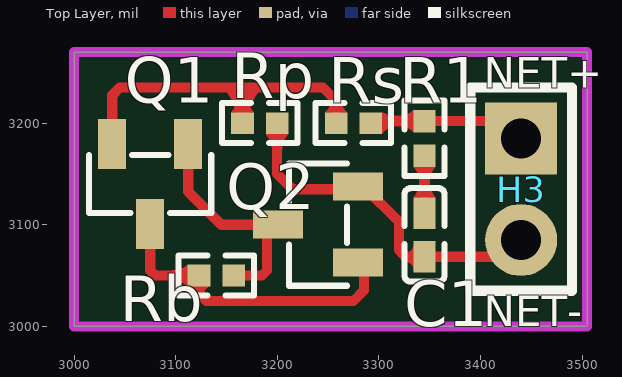
[diagram p0: Top Layer view]
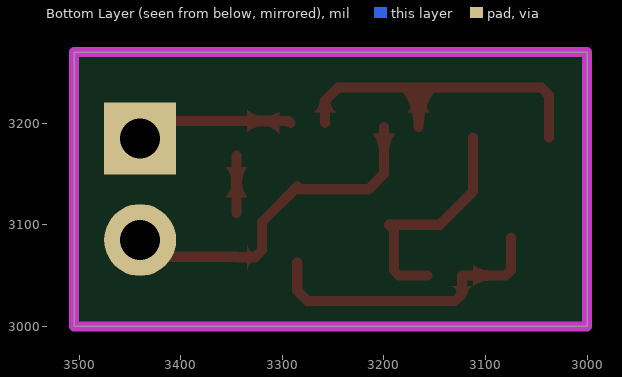
[diagram p1: Bottom Layer view, seen from below]
# Altium PCB MISC51453.pcbdoc
Units mil, origin at the board's own origin, x right, y up, seen from the top; angles counter-clockwise.
Board outline 505 x 270 mil, 2 copper layers (Top Layer, Bottom Layer), stack 62.206 mil thick; 8 components, 6 nets, 18 pads, 0 vias.

## Layer stack, top to bottom
Top Solder Mask Layer: solder mask 0.394, Dk 3.3
Top Layer: signal copper 1.379
Dielectric1: surface 59.449, FR4, Dk 4.5
Bottom Layer: signal copper 1.378
Bottom Solder Mask Layer: solder mask 0.394, Dk 3.3

## Board outline
3000,3270 3000,3000 3505,3000 3505,3270

## Design rules (kind name [scope] priority, off if disabled: settings)
BoardOutlineClearance copperThickness2oz_1 [All] p2 off: genericclearance=7.99 ignorepadtopadclearanceinfootprint=FALSE except(0: Arc-SplitContinuation Track-SplitContinuation SMDPad-SplitContinuation THPad-SplitContinuation Via-SplitContinuation Fill-SplitContinuation Region-SplitContinuation Poly-SplitContinuation Text-SplitContinuation Hole-SplitContinuation; 5.98: Arc-CutoutEdge Track-CutoutEdge SMDPad-CutoutEdge THPad-CutoutEdge Via-CutoutEdge Text-CutoutEdge; 6.9: Hole-OutlineEdge Hole-CutoutEdge; 10: Poly-OutlineEdge Poly-CutoutEdge; 11.81: Arc-OutlineEdge Track-OutlineEdge SMDPad-OutlineEdge THPad-OutlineEdge Via-OutlineEdge Fill-OutlineEdge Region-OutlineEdge Text-OutlineEdge Fill-CutoutEdge Region-CutoutEdge)
BoardOutlineClearance Plane_innerPlane_1 [All] p4 off: genericclearance=4.02 ignorepadtopadclearanceinfootprint=FALSE except(0: Arc-SplitContinuation Track-SplitContinuation SMDPad-SplitContinuation THPad-SplitContinuation Via-SplitContinuation Fill-SplitContinuation Region-SplitContinuation Poly-SplitContinuation Text-SplitContinuation Hole-SplitContinuation; 5.98: Arc-CutoutEdge Track-CutoutEdge SMDPad-CutoutEdge THPad-CutoutEdge Via-CutoutEdge Text-CutoutEdge; 6.9: Hole-OutlineEdge Hole-CutoutEdge; 10: Poly-OutlineEdge Poly-CutoutEdge; 11.81: Arc-OutlineEdge Track-OutlineEdge SMDPad-OutlineEdge THPad-OutlineEdge Via-OutlineEdge Fill-OutlineEdge Region-OutlineEdge Text-OutlineEdge Fill-CutoutEdge Region-CutoutEdge)
BoardOutlineClearance Copper_copperRegion_1 [All] p6 off: genericclearance=4.02 ignorepadtopadclearanceinfootprint=FALSE except(0: Arc-SplitContinuation Track-SplitContinuation SMDPad-SplitContinuation THPad-SplitContinuation Via-SplitContinuation Fill-SplitContinuation Region-SplitContinuation Poly-SplitContinuation Text-SplitContinuation Hole-SplitContinuation; 5.98: Arc-CutoutEdge Track-CutoutEdge SMDPad-CutoutEdge THPad-CutoutEdge Via-CutoutEdge Text-CutoutEdge; 6.9: Hole-OutlineEdge Hole-CutoutEdge; 10: Poly-OutlineEdge Poly-CutoutEdge; 11.81: Arc-OutlineEdge Track-OutlineEdge SMDPad-OutlineEdge THPad-OutlineEdge Via-OutlineEdge Fill-OutlineEdge Region-OutlineEdge Text-OutlineEdge Fill-CutoutEdge Region-CutoutEdge)
BoardOutlineClearance copperThickness1oz_1 [All] p8: genericclearance=4.02 ignorepadtopadclearanceinfootprint=FALSE except(0: Arc-SplitContinuation Track-SplitContinuation SMDPad-SplitContinuation THPad-SplitContinuation Via-SplitContinuation Fill-SplitContinuation Region-SplitContinuation Poly-SplitContinuation Text-SplitContinuation Hole-SplitContinuation; 5.98: Arc-CutoutEdge Track-CutoutEdge SMDPad-CutoutEdge THPad-CutoutEdge Via-CutoutEdge Text-CutoutEdge; 6.9: Hole-OutlineEdge Hole-CutoutEdge; 10: Poly-OutlineEdge Poly-CutoutEdge; 11.81: Arc-OutlineEdge Track-OutlineEdge SMDPad-OutlineEdge THPad-OutlineEdge Via-OutlineEdge Fill-OutlineEdge Region-OutlineEdge Text-OutlineEdge Fill-CutoutEdge Region-CutoutEdge)
Clearance copperThickness2oz [All] p1 off: gap=7.99 ignorepadtopadclearanceinfootprint=FALSE except(5.98: SMDPad-Track SMDPad-SMDPad THPad-Track SMDPad-THPad THPad-THPad Track-Via SMDPad-Via THPad-Via Via-Via Fill-SMDPad Region-SMDPad Fill-THPad Region-THPad Fill-Via Region-Via Fill-Fill Fill-Region Region-Region Arc-Track Arc-SMDPad Arc-THPad Arc-Via Fill-Arc Region-Arc Arc-Arc Text-Track SMDPad-Text Text-THPad Text-Via Fill-Text Region-Text Arc-Text Text-Text; 6.9: Hole-Track Hole-SMDPad Hole-THPad Hole-Via Fill-Hole Region-Hole Hole-Arc Hole-Text; 10: Poly-Track Poly-SMDPad Poly-THPad Poly-Via Poly-Fill Poly-Region Poly-Poly Poly-Arc Poly-Text Poly-Hole; 11.81: Fill-Track Region-Track)
Clearance Plane_innerPlane [All] p3 off: gap=4.02 ignorepadtopadclearanceinfootprint=FALSE except(5.98: SMDPad-Track SMDPad-SMDPad THPad-Track SMDPad-THPad THPad-THPad Track-Via SMDPad-Via THPad-Via Via-Via Fill-SMDPad Region-SMDPad Fill-THPad Region-THPad Fill-Via Region-Via Fill-Fill Fill-Region Region-Region Arc-Track Arc-SMDPad Arc-THPad Arc-Via Fill-Arc Region-Arc Arc-Arc Text-Track SMDPad-Text Text-THPad Text-Via Fill-Text Region-Text Arc-Text Text-Text; 6.9: Hole-Track Hole-SMDPad Hole-THPad Hole-Via Fill-Hole Region-Hole Hole-Arc Hole-Text; 10: Poly-Track Poly-SMDPad Poly-THPad Poly-Via Poly-Fill Poly-Region Poly-Poly Poly-Arc Poly-Text Poly-Hole; 11.81: Fill-Track Region-Track)
Clearance Copper_copperRegion [All] p5 off: gap=4.02 ignorepadtopadclearanceinfootprint=FALSE except(5.98: SMDPad-Track SMDPad-SMDPad THPad-Track SMDPad-THPad THPad-THPad Track-Via SMDPad-Via THPad-Via Via-Via Fill-SMDPad Region-SMDPad Fill-THPad Region-THPad Fill-Via Region-Via Fill-Fill Fill-Region Region-Region Arc-Track Arc-SMDPad Arc-THPad Arc-Via Fill-Arc Region-Arc Arc-Arc Text-Track SMDPad-Text Text-THPad Text-Via Fill-Text Region-Text Arc-Text Text-Text; 6.9: Hole-Track Hole-SMDPad Hole-THPad Hole-Via Fill-Hole Region-Hole Hole-Arc Hole-Text; 10: Poly-Track Poly-SMDPad Poly-THPad Poly-Via Poly-Fill Poly-Region Poly-Poly Poly-Arc Poly-Text Poly-Hole; 11.81: Fill-Track Region-Track)
Clearance copperThickness1oz [All] p7: gap=4.02 ignorepadtopadclearanceinfootprint=FALSE except(5.98: SMDPad-Track SMDPad-SMDPad THPad-Track SMDPad-THPad THPad-THPad Track-Via SMDPad-Via THPad-Via Via-Via Fill-SMDPad Region-SMDPad Fill-THPad Region-THPad Fill-Via Region-Via Fill-Fill Fill-Region Region-Region Arc-Track Arc-SMDPad Arc-THPad Arc-Via Fill-Arc Region-Arc Arc-Arc Text-Track SMDPad-Text Text-THPad Text-Via Fill-Text Region-Text Arc-Text Text-Text; 6.9: Hole-Track Hole-SMDPad Hole-THPad Hole-Via Fill-Hole Region-Hole Hole-Arc Hole-Text; 10: Poly-Track Poly-SMDPad Poly-THPad Poly-Via Poly-Fill Poly-Region Poly-Poly Poly-Arc Poly-Text Poly-Hole; 11.81: Fill-Track Region-Track)
DiffPairsRouting differentialPair [All] p1: maxlimit=6 minlimit=6 mostfreqgap=6 toplayer_minwidth=5 toplayer_prefwidth=10 toplayer_maxwidth=100 toplayer_mingap=6 toplayer_prefgap=6 toplayer_maxgap=6 bottomlayer_minwidth=5 bottomlayer_prefwidth=10 bottomlayer_maxwidth=100 bottomlayer_mingap=6 bottomlayer_prefgap=6 bottomlayer_maxgap=6 maxuncoupledlength=10
HoleToHoleClearance otherClearance [All] p1: gap=11.81 allowstackedmicrovias=TRUE
Length netLength [All] p1: minlimit=0 maxlimit=0
PasteMaskExpansion pasteMaskExpansion [All] p1: expansion=0
PlaneConnect innerPlane [All] p1: planeconnectstyle=Relief reliefexpansion=20 reliefentries=4 reliefconductorwidth=10 reliefairgap=10
PolygonConnect copperRegion [All] p1: connectstyle=Relief reliefconductorwidth=10 reliefentries=4 polygonreliefangle="90 Angle" airgapwidth=10 via.connectstyle=Relief via.reliefconductorwidth=10 via.reliefentries=4 via.polygonreliefangle="90 Angle" via.airgapwidth=10
RoutingVias viaSize [All] p1: holewidth=12.01 width=24.02 viastyle="Through Hole" minholewidth=11.81 minwidth=19.68 maxholewidth=248.03 maxwidth=393.7
SolderMaskExpansion solderMaskExpansion [IsVia] p1: expansion=-1000 istentingtop=TRUE
SolderMaskExpansion solderMaskExpansion [All] p2: expansion=2 istentingtop=FALSE
Width copperThickness2oz_2 [All] p1 off: maxlimit=100 minlimit=8 preferedwidth=10
Width copperThickness1oz_2 [All] p2: maxlimit=100 minlimit=5 preferedwidth=10

## Components (designator, comment, footprint, x,y, rotation, side; value= is the part's Value field where it differs from the comment)
C1 "10uF" C0402 3345,3090 r90 top
H3 "" HDR-TH_2P-P2.54-V-M-1 3440,3135 r270 top
Q1 "MMBT3906" SOT-23-3_L2.9-W1.3-P1.90-LS2.4-BR 3075,3140 r90 top
Q2 "MMBT3904" SOT-23-3_L2.9-W1.3-P1.90-LS2.4-BR 3240,3100 r0 top
R1 "0" R0402 3345,3185 r90 top
Rb "1K" R0402 3140,3050 r0 top
Rp "200K" R0402 3182.83,3200 r180 top
Rs "200" R0402 3275,3200 r0 top

## Footprints (in the part's own frame and the unit in brackets; to place one, negate y for a bottom-side part, rotate by r counter-clockwise, add the part's x,y. Pads: shape width x height; smd on the part's side, far side on the other; paste and mask are expansions set on the pad)
C0402 [mm]
  rect 0.79x0.54 smd paste-100 mask+0.051: 1(-0.545,0) 2(0.545,0)
  silkscreen extent -1.17,-0.5 1.17,0.5
HDR-TH_2P-P2.54-V-M-1 [mm]
  rect 1.8x1.8 hole 1: 1(-1.27,0)
  round 1.8 hole 1: 2(1.27,0)
  silkscreen extent -2.54,-1.27 2.54,1.27
R0402 [mm]
  rect 0.566x0.54 smd paste-100 mask+0.051: 1(-0.433,0) 2(0.433,0)
  silkscreen extent -0.94,-0.5 0.94,0.5
SOT-23-3_L2.9-W1.3-P1.90-LS2.4-BR [mm]
  rect 1.25x0.7 smd: 1(1,-0.95) 2(1,0.95) 3(-1,0)
  silkscreen extent -0.73,-1.53 0.73,1.53

## Nets (pads, with @x,y where several pads share a name; then routed paths per layer and width w, separated by ;. In a path a pad name is that pad's centre, name@x,y a point inside that pad or via, vN(x,y) a via of type N, cw(c..) or ccw(c..) an arc to the next point about the centre after c; other vN are vias at no path point)
$1N1099: Q1.2 Rp.2 Rs.1 | length 332.2
  Top Layer w10: Q1.2@3037.6,3185.84 3037.6,3227.6 3045,3235 3167.98,3235 ; Rp.2@3165.79,3196.32 3165.79,3232.81 3167.98,3235 ; Rs.1 3257.96,3222.04 3245,3235 3167.98,3235
$1N1121: C1.2 R1.1 | length 56.5
  Top Layer w10: C1.2 R1.1
$1N1168: Q1.1 Q2.3 Rb.2 | length 231.1
  Top Layer w10: Q1.1@3112.4,3185.84 3112.4,3132.6 3145,3100 3194.72,3100 3190,3095.28 3190,3055 3185,3050 Rb.2
$1N1173: Q1.3 Q2.1 Rb.1 | length 297.2
  Top Layer w10: Q1.3@3075,3087.44 3075,3055 3080,3050 Rb.1 3122.96,3032.04 3130,3025 3275,3025 3285.28,3035.28 Q2.1@3285.28,3062.6
NET+: H3.1 R1.2 Rs.2 | length 155.9
  Top Layer w10: Rs.2 3294.08,3202.04 R1.2 3422.96,3202.04 H3.1
NET-: C1.1 H3.2 Q2.2 Rp.1 | length 345.6
  Top Layer w10: Rp.1@3199.87,3196.32 3199.87,3150.13 3215,3135 3282.87,3135 3285.28,3137.4 3320,3102.68 3320,3075 3327.07,3067.93 3344.39,3067.93 C1.1 3423.54,3068.54 H3.2

## Keep-outs
Board Outline Layer:
  the board outline again, w10

## Other copper
Top Layer:
  region net $1N1121: 3340,3142.01 3350,3142.01 3350.37,3137.94 3351.45,3134 3353.23,3130.32 3355.63,3127.01 3334.37,3127.01 3336.77,3130.32 3338.55,3134 3339.63,3137.94 3340,3142.01
  region net NET-: 3327.07,3062.93 3327.07,3072.93 3329.34,3073.35 3331.38,3074.43 3332.98,3076.09 3334.02,3078.15 3334.37,3080.43 3334.37,3055.43 3334.02,3057.71 3332.98,3059.77 3331.38,3061.43 3329.34,3062.51 3327.07,3062.93
  region net NET+: 3319.37,3197.04 3319.37,3207.04 3322.68,3207.3 3325.91,3208.06 3328.99,3209.32 3331.83,3211.04 3334.37,3213.18 3334.37,3190.91 3331.83,3193.04 3328.99,3194.76 3325.91,3196.02 3322.68,3196.78 3319.37,3197.04
  region net $1N1121: 3350,3141.82 3340,3141.82 3339.63,3145.9 3338.55,3149.84 3336.77,3153.52 3334.37,3156.82 3355.63,3156.82 3353.23,3153.52 3351.45,3149.84 3350.37,3145.9 3350,3141.82
  region net $1N1173: 3096.82,3045 3096.82,3055 3100.9,3055.37 3104.84,3056.45 3108.52,3058.23 3111.82,3060.63 3111.82,3039.37 3108.52,3041.77 3104.84,3043.55 3100.9,3044.63 3096.82,3045
  region net $1N1173: 3127.96,3032.04 3117.96,3032.04 3117.67,3034.09 3116.83,3035.98 3115.5,3037.57 3113.79,3038.73 3111.82,3039.37 3134.09,3039.37 3132.13,3038.73 3130.42,3037.57 3129.09,3035.98 3128.25,3034.09 3127.96,3032.04
  region net $1N1099: 3160.79,3225.63 3170.79,3225.63 3171.04,3222.32 3171.81,3219.09 3173.07,3216.01 3174.79,3213.17 3176.92,3210.63 3154.65,3210.63 3156.79,3213.17 3158.51,3216.01 3159.76,3219.09 3160.53,3222.32 3160.79,3225.63
  region net NET-: 3204.87,3174.37 3194.87,3174.37 3194.61,3177.68 3193.84,3180.91 3192.59,3183.99 3190.87,3186.83 3188.73,3189.37 3211,3189.37 3208.87,3186.83 3207.15,3183.99 3205.89,3180.91 3205.12,3177.68 3204.87,3174.37
  region net NET+: 3318.18,3207.04 3318.18,3197.04 3314.72,3196.72 3311.38,3195.76 3308.27,3194.21 3305.51,3192.11 3303.18,3189.54 3303.18,3210.63 3306.74,3209.08 3310.46,3207.95 3314.29,3207.27 3318.18,3207.04
  region net $1N1099: 3252.96,3222.04 3262.96,3222.04 3263.23,3219.36 3264.01,3216.78 3265.29,3214.41 3267,3212.33 3269.09,3210.63 3246.82,3210.63 3248.92,3212.33 3250.63,3214.41 3251.91,3216.78 3252.69,3219.36 3252.96,3222.04
  region net $1N1099: 3160.79,3200 3160.5,3205.35 3159.64,3210.64 3158.22,3215.81 3156.26,3220.8 3153.77,3225.55 3150.79,3230 3167.98,3235 3180.79,3230 3177.8,3225.55 3175.32,3220.8 3173.35,3215.81 3171.93,3210.64 3171.07,3205.35 3170.79,3200

## Silkscreen, mask and mechanical layers (free items; w line width, h text height)
Top Silkscreen Layer:
  text "NET+" at 3403.05,3235 h30
  text "NET-" at 3403.05,3000 h30